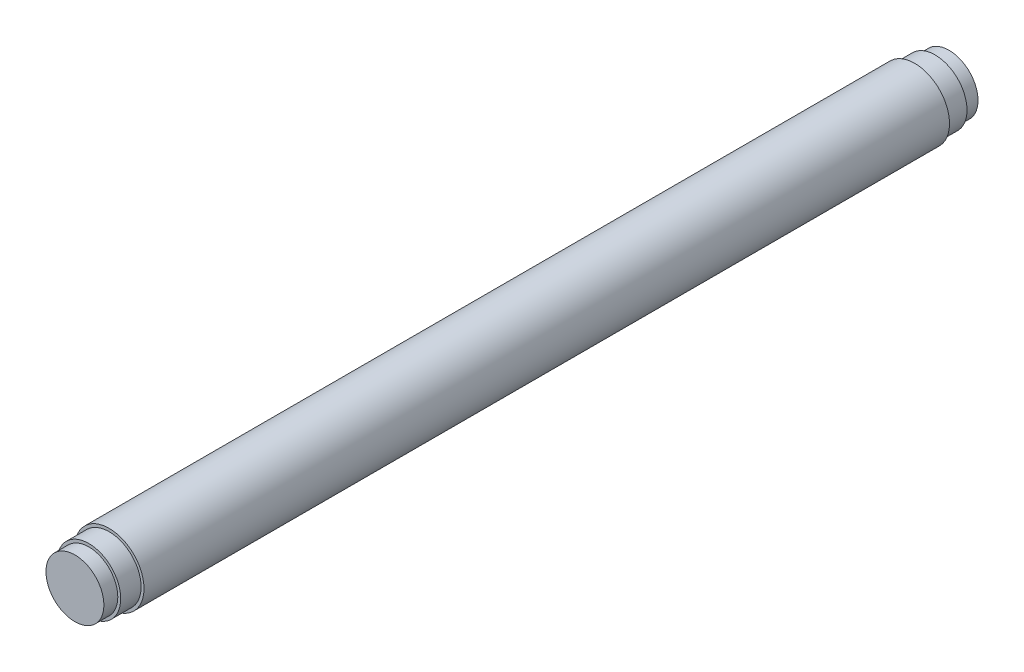
from build123d import *

# Parameters (mm, degrees)
SKETCH1_R           = 27.5
BOSS_EXTRUDE1_DEPTH = 17.6
SKETCH2_R           = 25
BOSS_EXTRUDE2_DEPTH = 12
SKETCH3_R           = 30
BOSS_EXTRUDE3_DEPTH = 695
SKETCH4_R           = 27.5
BOSS_EXTRUDE4_DEPTH = 17.6
BOSS_EXTRUDE5_START = 12
SKETCH5_R           = 25
BOSS_EXTRUDE5_DEPTH = 12


with BuildPart() as part:
    # Sketch1 → Boss-Extrude1 (new body)
    with BuildSketch(Plane.XY):
        Circle(SKETCH1_R)
    extrude(amount=BOSS_EXTRUDE1_DEPTH)

    # Sketch2 → Boss-Extrude2 (add)
    with BuildSketch(Plane(origin=(0, 0, 0), x_dir=(-1, 0, 0), z_dir=(0, 0, -1))):
        with Locations(Location((0, 0, 0), (0, 0, 180))):
            Circle(SKETCH2_R)
    extrude(amount=BOSS_EXTRUDE2_DEPTH)

    # Sketch3 → Boss-Extrude3 (add)
    with BuildSketch(Plane.XY.offset(17.6)):
        Circle(SKETCH3_R)
    extrude(amount=BOSS_EXTRUDE3_DEPTH)

    # Sketch4 → Boss-Extrude4 (add)
    with BuildSketch(Plane.XY.offset(712.6)):
        Circle(SKETCH4_R)
    extrude(amount=BOSS_EXTRUDE4_DEPTH)

    # Sketch5 → Boss-Extrude5 (add)
    with BuildSketch(Plane.XY.offset(730.2).offset(BOSS_EXTRUDE5_START)):
        Circle(SKETCH5_R)
    extrude(amount=-BOSS_EXTRUDE5_DEPTH)


solid = part.part
